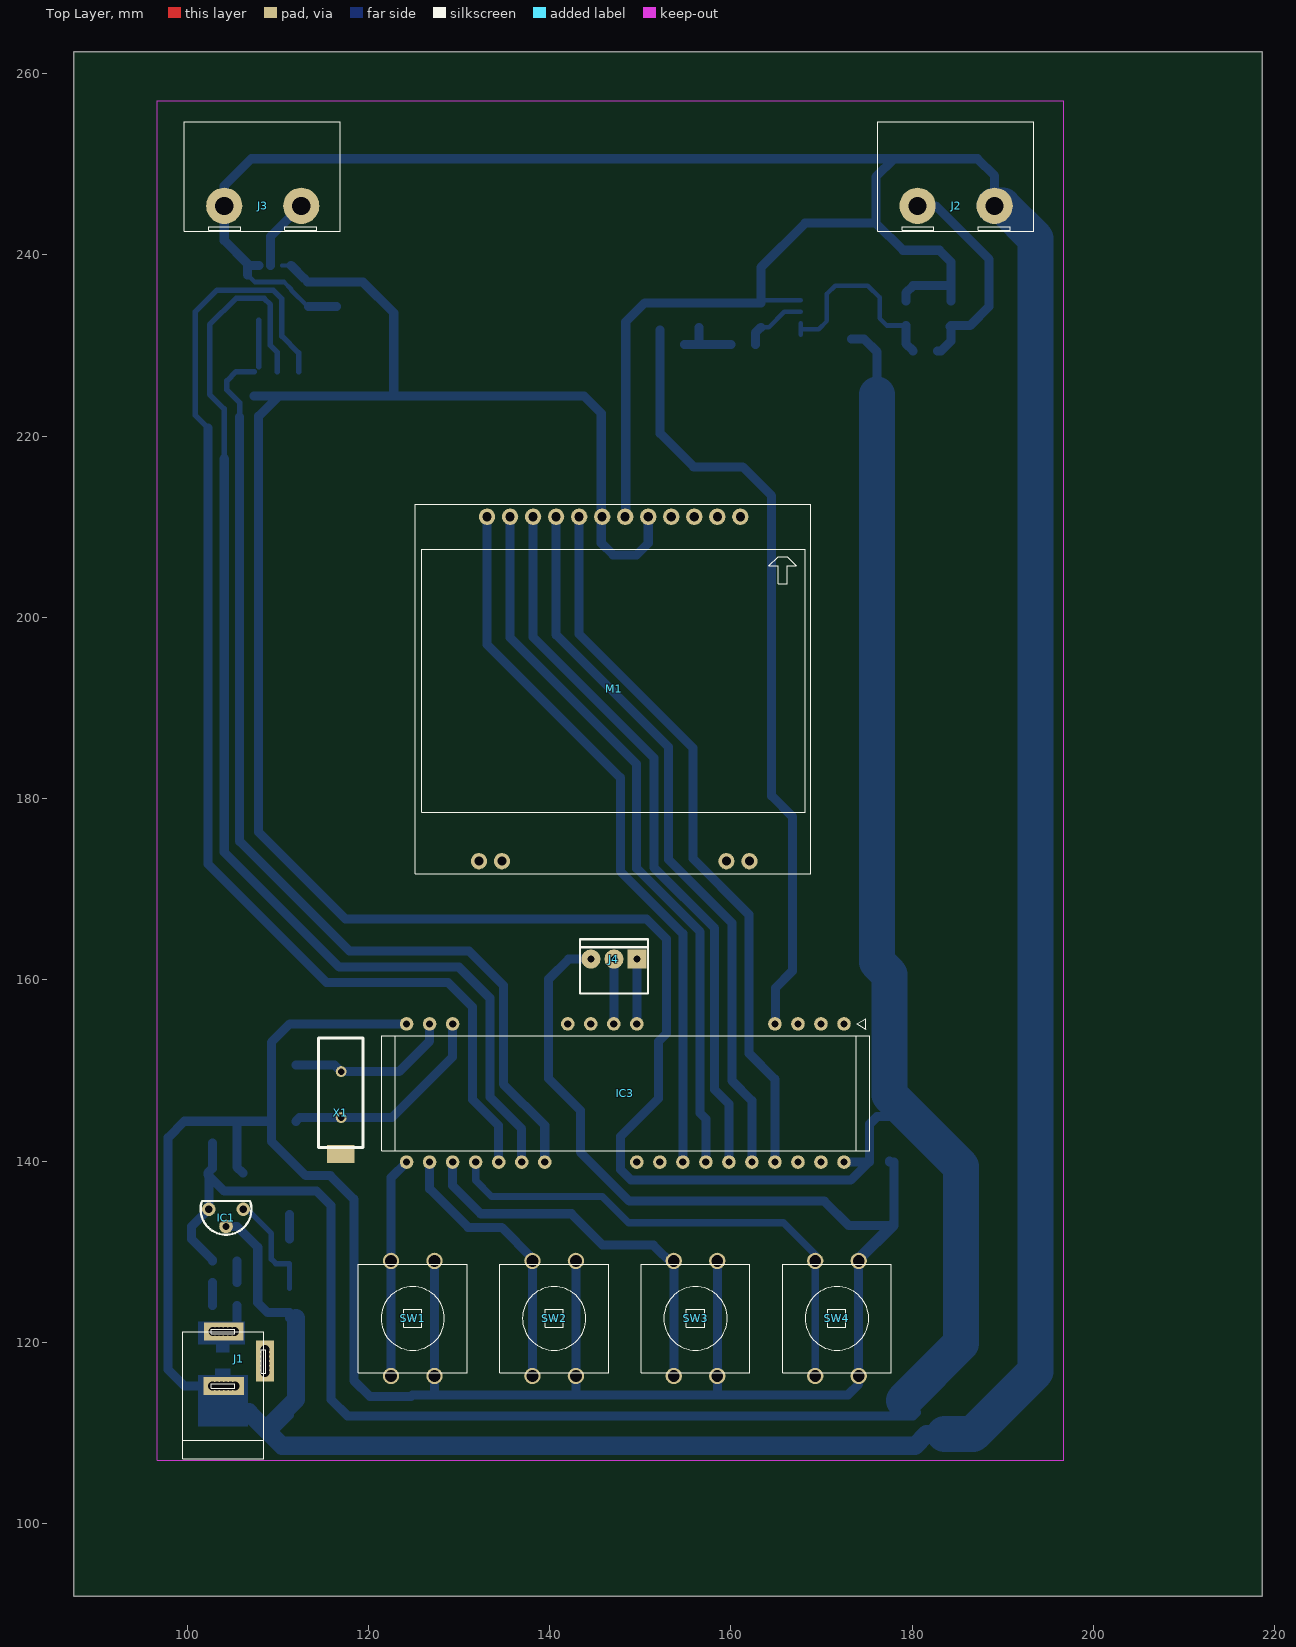
[diagram p0: Top Layer view]
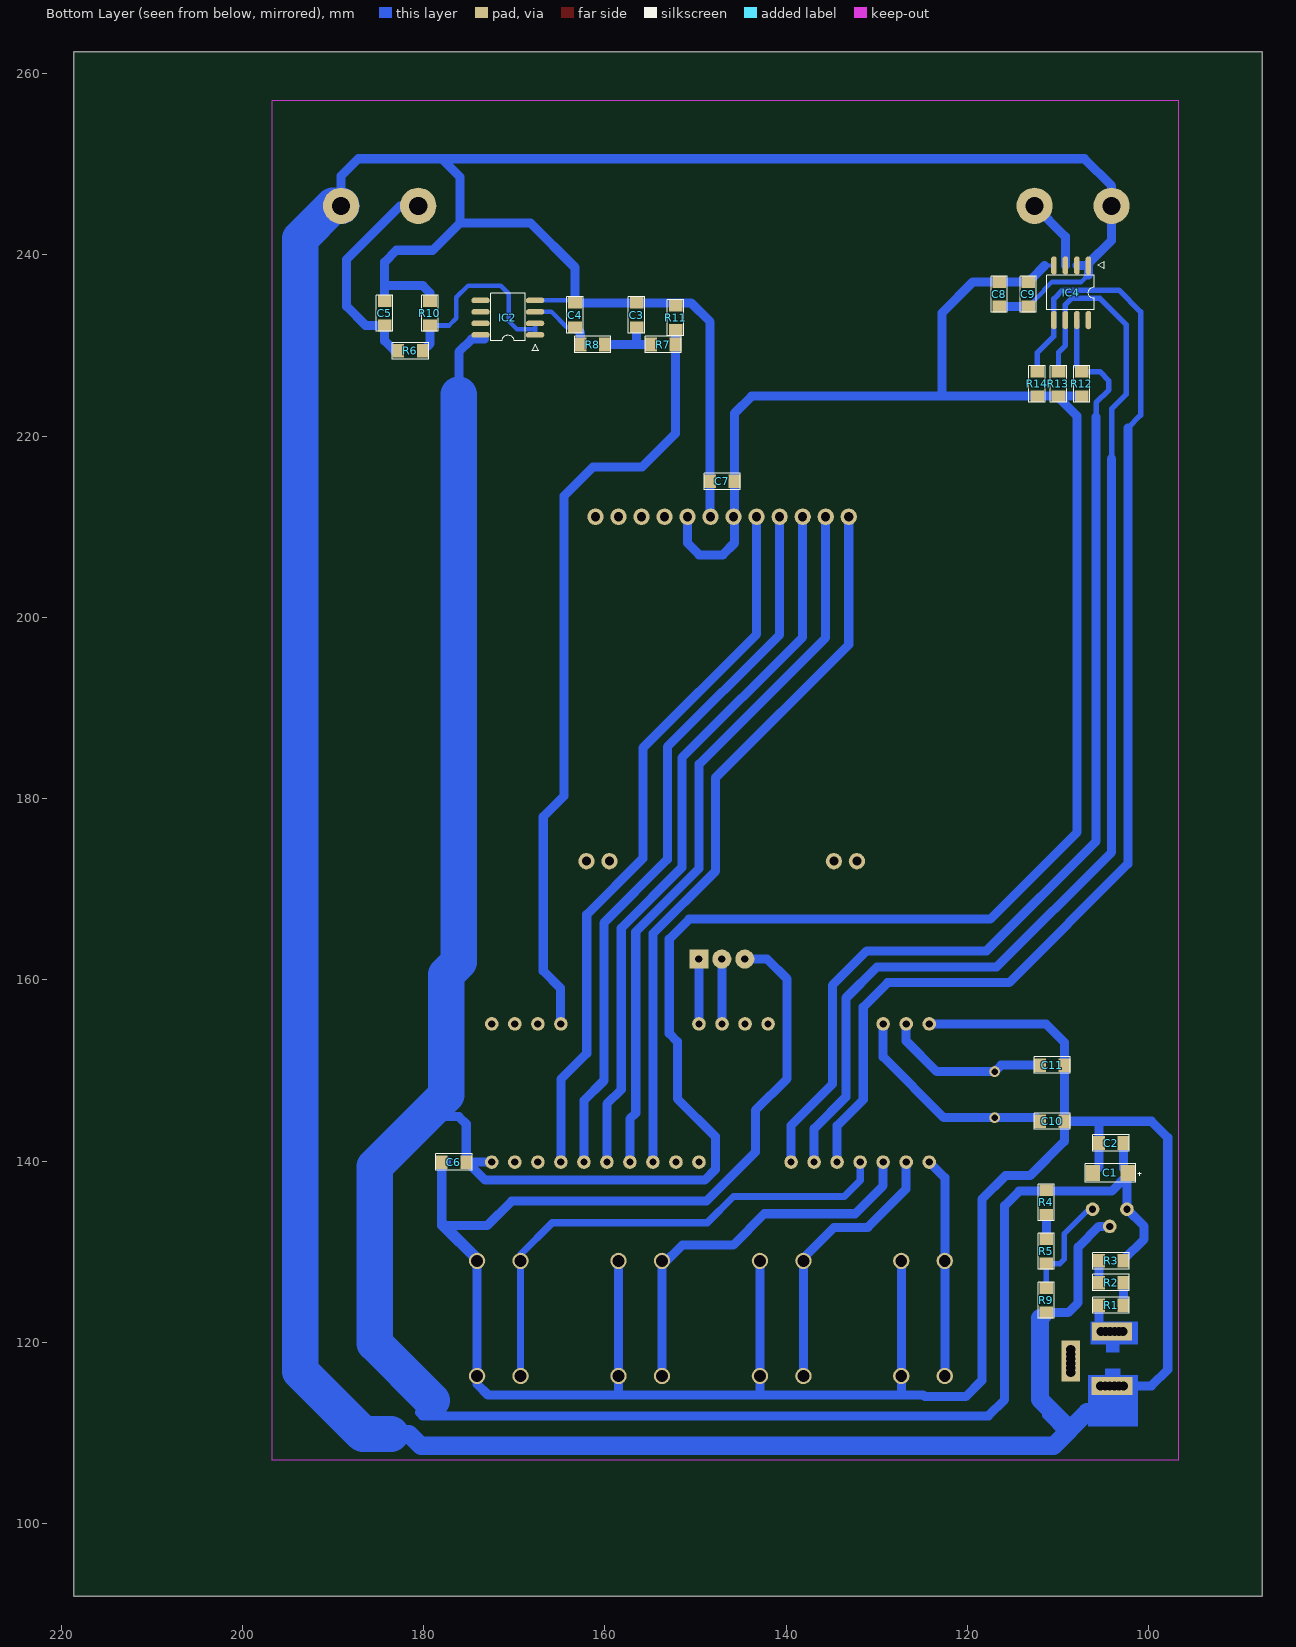
[diagram p1: Bottom Layer view, seen from below]
# Altium PCB MISC82230.PcbDoc
Units mm, origin at the board's own origin, x right, y up, seen from the top; angles counter-clockwise.
Board outline 131.1 x 170.4 mm, 2 copper layers (Top Layer, Bottom Layer); 39 components, 30 nets, 157 pads, 0 vias.

## Layer stack, top to bottom (the 12.6 mil dielectric is the usual default, probably not edited)
Top Layer: signal copper 0.0356
Dielectric: dielectric 0.32, FR-4, Dk 4.8
Bottom Layer: signal copper 0.0356

## Board outline
87.9,262.4 218.6,262.4 218.6,92 87.5,92 87.5,99.3 87.5,262.4 87.9,262.4

## Design rules (kind name [scope] priority, off if disabled: settings)
Clearance [All] p1: gap=0.2
ComponentClearance [All] p1: gap=0.254 collisioncheckmode=3 verticalgap=0.254
PolygonConnect [All] p1: connectstyle=Relief reliefconductorwidth=0.254 reliefentries=4 polygonreliefangle="90 Angle"
RoutingVias [All] p1: holewidth=0.711 width=1.27 viastyle="Through Hole" minholewidth=0.711 minwidth=1.27 maxholewidth=9 maxwidth=9
SolderMaskExpansion [All] p1: expansion=0.102
TestPointUsage [All] p1: valid=0 allowmultiple=FALSE
Testpoint [All] p1: side=15 testpointundercomponent=TRUE minsize=1.016 maxsize=2.54 preferedsize=1.524 minholesize=0 maxholesize=1.016 preferedholesize=0.813 testpointgrid=0.025 style=1023 order=0-112345678
Width [All] p1: maxlimit=9 minlimit=0.254 preferedwidth=0.3
18 further rules are at their usual default settings.

## Classes and differential pairs
component class Sheet1: C1 C2 C5 C6 C7 C8 C9 C10 C11 IC1 IC3 IC4 J1 J2 J3 J4 M1 R1 R2 R3 R4 R5 R8 R9 R10 R11 R12 R13 R14 SW1 SW2 SW3 SW4 X1

## Components (designator, comment, footprint, x,y, rotation, side; value= is the part's Value field where it differs from the comment)
C1 "10UF" C10 103.9,139.1 r0 bottom
C2 "104" 0805 102.8,142.001 r0 bottom
C3 "104" 0805 156.5,232 r90 bottom
C4 "104" 0805 163.299,232 r90 bottom
C5 "106" 0805 184.3,232.2 r90 bottom
C6 "106" 0805 175.3,139.9 r0 bottom
C7 "104" 0805 145.7,215.001 r0 bottom
C8 "106" 0805 116.5,237 r270 bottom
C9 "104" 0805 113.3,237 r270 bottom
C10 "22P" 0805 112,144.4 r180 bottom
C11 "22P" 0805 112,150.599 r180 bottom
IC1 "TL431" TO92 106.2,134.7 r180 top
IC2 "LM358/rail-to-rail" SOP8 167.675,231.13 r0 bottom
IC3 "12C5A60S2" DIP40 172.48,155.14 r180 top locked
IC4 "MAX6675" SOP8 106.63,238.845 r270 bottom
J1 "J3/5V/DC/POW" DC/POW 108.45,121.2 r270 top
J2 "0.8--4.6" SIP2/8.5 189.1,245.4 r180 top
J3 "K/IN" SIP2/8.5 112.6,245.4 r180 top
J4 "ISP" SIP3 149.156,162.511 r180 top
M1 "S/12864/LCD" S/12864/LCD 125.2,171.7 r0 top
R1 "1" 0805 102.8,124.1 r0 bottom
R2 "1" 0805 105.5,126.6 r180 bottom
R3 "1" 0805 102.8,129 r0 bottom
R4 "10" 0805 111.301,136.8 r270 bottom
R5 "10K" 0805 111.301,131.4 r270 bottom
R6 "1K" 0805 180.1,229.401 r0 bottom
R7 "10K" 0805 152.2,230.1 r0 bottom
R8 "10K" 0805 160,230.101 r0 bottom
R9 "10K" 0805 111.301,126 r270 bottom
R10 "10K" 0805 179.301,234.9 r270 bottom
R11 "100K" 0805 152.201,234.4 r270 bottom
R12 "10K" 0805 107.399,224.4 r90 bottom
R13 "10K" 0805 109.957,224.4 r90 bottom
R14 "10K" 0805 112.315,224.4 r90 bottom
SW1 "A" BUTTON/B 122.5,129 r0 top
SW2 "B" BUTTON/B 138.1,129 r0 top
SW3 "-" BUTTON/B 153.7,129 r0 top
SW4 "+" BUTTON/B 169.3,129 r0 top
X1 "12M" X 117,144.8 r90 top

## Footprints (in the part's own frame and the unit in brackets; to place one, negate y for a bottom-side part, rotate by r counter-clockwise, add the part's x,y. Pads: shape width x height; smd on the part's side, far side on the other; paste and mask are expansions set on the pad)
0805 [mm]
  rect 1.3x1.5 smd: 1(0,0) 2(2.7,0.001)
  silkscreen extent -0.65,-0.9 3.35,0.9
BUTTON/B [mm]
  round 1.8 hole 1.3: 1(0,-12.7) 1(0,0) 2(4.8,-12.7) 2(4.8,0)
  silkscreen extent -3.6,-12.35 8.4,-0.35
C10 [mm]
  rect 1.6x1.8 smd: 1(-1.6,0.4) 2(2.25,0.4)
  silkscreen extent -3.1,-0.59 3.1,1.41
DC/POW [mm]
  rect 2x2 hole 1: 1(0,-3.2) 1(0,-3.7) 1(0,-4.2) 1(0,-4.7) 1(0,-5.15) 1(0,-5.6) 2(6,-5.65) 2(6,-5.15) 2(6,-4.65) 2(6,-4.15) 2(6,-3.65) 2(6,-3.15) 3(2,0.15) 3(2.5,0.15) 3(3,0.15) 3(3.5,0.15) 3(4,0.15) 3(4.5,0.15)
  silkscreen extent -0.25,-8.95 14.05,0.25
DIP40 [mm]
  round 1.5 hole 0.8: 1(0,0) 2(2.54,0) 3(5.08,0) 4(7.62,0) 10(22.86,0) 11(25.4,0) 12(27.94,0) 13(30.48,0) 18(43.18,0) 19(45.72,0) 20(48.26,0) 21(48.26,15.24) 22(45.72,15.24) 23(43.18,15.24) 24(40.64,15.24) 25(38.1,15.24) 26(35.56,15.24) 27(33.02,15.24) 31(22.86,15.24) 32(20.32,15.24) 33(17.78,15.24) 34(15.24,15.24) 35(12.7,15.24) 36(10.16,15.24) 37(7.62,15.24) 38(5.08,15.24) 39(2.54,15.24) 40(0,15.24)
  silkscreen extent -2.85,-0.6 51,13.99
S/12864/LCD [mm]
  round 1.8 hole 1: 1(35.84,39.4) 2(33.3,39.4) 3(30.76,39.4) 4(28.22,39.4) 5(25.68,39.4) 6(23.14,39.4) 7(20.6,39.4) 8(18.06,39.4) 9(15.52,39.4) 10(12.98,39.4) 11(10.44,39.4) 12(7.9,39.4) 13(7,1.4) 14(9.54,1.4) 15(34.3,1.4) 16(36.84,1.4)
  silkscreen extent 0,0 43.6,40.8
SIP2/8.5 [mm]
  round 4 hole 2: 1(0,0) 2(8.5,0)
  silkscreen extent -4.3,-9.3 12.9,2.8
SIP3 [mm]
  rect 2.1x2.1 hole 0.813: 1(-0.484,0.211)
  round 2.1 hole 0.813: 2(2.056,0.211) 3(4.596,0.211)
  silkscreen extent -1.7,-1.99 5.8,4.01
SOP8 [mil]
  oval 80x24 smd: 1(0.99,-1.18) 2(0.99,-51.18) 3(0.99,-101.18) 4(0.99,-151.18) 5(237.99,-151.18) 6(237.99,-101.18) 7(237.99,-51.18) 8(237.99,-1.18)
  silkscreen extent -16,-181 194,67
TO92 [mm]
  round 1.5 hole 0.8 unplated: 1(0,0) 2(1.9,1.9) 3(3.8,0)
  silkscreen extent -0.9,-0.9 4.7,2.81
X [mm]
  round 1.2 hole 0.7: 1(0,0) 2(5.08,0)
  rect 2x3 smd: 3(-4.009,0.042)
  silkscreen extent -3.3,-2.4 8.78,2.5

## Part data
C1 C2 C3 C4 C5 C6 C7 C8 C9 C10 C11: library part C
IC1 IC2: library part LM358
IC3: library part 12C5A08AD
J1: library part DC/POW
J2 J3: library part J2
J4: library part J3
R1 R2 R3 R4 R5 R6 R7 R8 R9 R10 R11 R12 R13 R14: library part R
SW1 SW2 SW3 SW4: library part SW2
X1: library part X

## Nets (pads, with @x,y where several pads share a name; then routed paths per layer and width w, separated by ;. In a path a pad name is that pad's centre, name@x,y a point inside that pad or via, vN(x,y) a via of type N, cw(c..) or ccw(c..) an arc to the next point about the centre after c; other vN are vias at no path point)
0.8--4.6: C5.1 J2.2 R6.2 | length 24.4
  Bottom Layer w1: J2.2 182.6,245.4 188.5,239.5 188.5,234.3 186.4,232.2 C5.1 ; R6.2 183.2,229.4 184.3,230.5 C5.1 ; C5.1@184.2,232.1 C5.1
5.2V: J1.1 R1.2 | length 3.2
  Bottom Layer w1: J1.1@104.75,121.2 105.5,121.95 R1.2
5V: C1.1 C2.1 C6.1 C7.1 C8.1 C9.1 IC1.3 IC2.8 IC3.40 IC4.4 M1.5 M1.7 R3.1 R4.1 R12.1 R13.1 R14.1 | length 495.4
  Bottom Layer w0.4: IC4.4 111.48,238.82 ; M1.7@145.7,211.2 M1.7
  Bottom Layer w1: R3.1 102.8,129.1 100.5,131.4 100.5,132.8 IC1.3 102.4,138.6 C1.1 ; C2.1 102.8,139.2 C1.1 ; R12.1 R13.1@109.957,224.4 ; 111.48,238.82 C9.1@112.927,237.373 ; C9.1 119.4,237 122.8,233.6 122.8,224.4 ; M1.5 150.88,208.18 149.6,206.9 147,206.9 145.7,208.2 145.7,222.5 143.8,224.4 110.1,224.4 107.9,222.2 107.9,176.3 117.5,166.7 150.7,166.7 152.9,164.5 152.9,154.1 152,153.2 152,146.9 147.8,142.7 147.8,139.1 149,137.9 173.2,137.9 C6.1@175.2,139.9 ; IC3.40 C6.1 175.3,144.1 176.12,144.92 179.88,144.92 ; 173.3,230.7 174.7,230.7 176.12,229.28 176.12,224.6 ; 180.45,112.25 180.1,111.9 117.7,111.9 115.9,113.7 115.9,135.1 114.3,136.7 104.1,136.7 102.3,138.5 C1.1
  Bottom Layer w4: 176.12,224.6 176.12,161.98 177.5,160.6 177.5,147.3 185.4,139.4 185.4,119.9 179.1,113.6
GND: C1.2 C2.2 C3.2 C4.2 C5.2 C6.2 C7.2 C8.2 C9.2 C10.2 C11.2 IC1.2 IC2.4 IC3.20 IC4.1 IC4.2 J1.2 J2.1 J3.2 J4.3 M1.6 R9.2 R10.1 R11.1 SW1.2 SW2.2 SW3.2 SW4.2 | length 764
  Bottom Layer w0.5: 106.66,237.8 107.46,237 110.7,237 111.5,236.2 111.5,236.1 C9.2 C9.2@113.4,234.3 ; C4.2@163.57,234.97 IC2.4
  Bottom Layer w1: J1.2@103.3,115.2 99.7,115.2 97.9,117 97.9,142.6 99.701,144.401 C10.2 ; IC1.2 105.5,132.8 107.8,130.5 107.8,124.4 108.9,123.3 R9.2 R9.2@111.3,122.7 ; 105.5,144.301 105.5,139.35 C1.2 ; 106.66,237.8 IC4.1 ; IC4.2 IC4.1 ; 109.2,109.9 111.3,112 111.3,113 ; C9.2@113.4,234.3 C8.2 ; IC3.20 111.34,155.14 109.3,153.1 C10.2 ; SW1.2@127.3,129 127.3,114.3 127.4,114.2 ; 142.9,114.3 SW2.2@142.9,129 ; J4.3 142.1,162.3 139.9,160.1 139.9,149.1 143.4,145.6 143.4,141 148.8,135.6 170.3,135.6 173,132.9 178,132.9 ; M1.6 148.4,211.16 148.4,232.6 150.5,234.7 C4.2@163.3,234.7 ; 158.5,114.3 SW3.2@158.5,129 ; C4.2@163.3,235.24 163.3,238.6 168.2,243.5 176,243.5 ; SW4.2@174.1,129.4 178,133.3 ; C6.2@177.5,139.899 C6.2@177.5,140 ; C6.2 178,132.9 ; 178,250.6 176,248.6 176,243.5 ; R10.1 179.301,235.801 180.1,236.6 184.301,236.6 ; C5.2 184.301,239.199 183,240.5 179,240.5 176,243.5 ; J2.1 189.1,248.7 187.2,250.6 107.1,250.6 104.1,247.6 J3.2 104.1,241.6 106.66,239.04 IC4.1 ; C10.2 109.3,142.2 113.1,138.4 115.8,138.4 118.4,135.8 118.4,115.8 120.186,114.014 124.7,114.014 124.886,114.2 172.9,114.2 174.1,115.4 174.1,129 178,132.9
  Bottom Layer w2: 106.1,112.3 106.8,112.3 110.5,108.6 180.3,108.6 181.6,109.9 184.4,109.9 ; 108.9,110.4 108.9,110.6 112,113.7 R9.2@112,122.7
  Bottom Layer w4: 183.6,109.9 186.7,109.9 193.6,116.8 193.6,241.8 190,245.4 J2.1
K/CS: IC3.26 IC4.6 R13.2 | length 130.3
  Bottom Layer w0.6: 104.1,217.5 104.1,223 102.5,224.6 102.5,232.3 105.4,235.2 108.5,235.2 109.2,234.5 109.2,230 109.958,229.242 R13.2
  Bottom Layer w1: 104.1,217.5 104.1,174.1 116.8,161.4 130,161.4 133.4,158 133.4,147.1 136.92,143.58 IC3.26
K/SCK: IC3.25 IC4.5 R14.2 | length 135.3
  Bottom Layer w0.6: 102.3,220.9 100.9,222.3 100.9,233.7 103.3,236.1 109.5,236.1 110.47,235.13 110.47,231.03 112.316,229.184 R14.2
  Bottom Layer w1: 102.3,220.9 102.3,172.8 115.4,159.7 128.8,159.7 131.5,157 131.5,146.8 134.38,143.92 IC3.25
K/SO: IC3.27 IC4.7 R12.2 | length 117
  Bottom Layer w0.6: 105.8,222.1 105.8,223.7 104.4,225.1 104.4,226.1 105.4,227.1 R12.2 ; R12.2@107.93,227.63 IC4.7
  Bottom Layer w1: 105.8,222.1 105.8,175.3 117.9,163.2 131.1,163.2 134.9,159.4 134.9,148.5 139.46,143.94 IC3.27
KEY1: IC3.21 SW1.1 | length 24.3
  Bottom Layer w1: SW1.1@122.5,116.3 122.5,138.18 IC3.21
KEY2: IC3.22 SW2.1 | length 30.5
  Bottom Layer w1: IC3.22 126.76,136.94 131,132.7 134.7,132.7 138.1,129.3 SW2.1@138.1,116.3
KEY3: IC3.23 SW3.1 | length 42.8
  Bottom Layer w1: IC3.23 129.3,137.3 132.4,134.2 142.4,134.2 145.857,130.743 151.457,130.743 153.7,128.5 SW3.1@153.7,116.3
KEY4: IC3.24 SW4.1 | length 56.3
  Bottom Layer w0.8: IC3.24 131.84,137.86 133.6,136.1 145.8,136.1 148.7,133.2 165.8,133.2 169.3,129.7 SW4.1@169.3,116.3
LCD/BL: IC3.38
LCD/CS: IC3.33 M1.12 | length 80.1
  Bottom Layer w1: M1.12 133.1,197 147.8,182.3 147.8,172 154.7,165.1 IC3.33
LCD/RS: IC3.35 M1.10 | length 80.1
  Bottom Layer w1: M1.10 138.18,197.82 151.5,184.5 151.5,172.4 158.2,165.7 158.2,147.9 159.78,146.32 IC3.35
LCD/RST: IC3.34 M1.11 | length 80.1
  Bottom Layer w1: M1.11 135.64,197.76 149.6,183.8 149.6,172.3 156.6,165.3 156.6,145.3 157.24,144.66 IC3.34
LCD/SCK: IC3.37 M1.8 | length 80.1
  Bottom Layer w1: M1.8 143.26,198.14 155.8,185.6 155.8,173.4 162,167.2 162,151.9 164.86,149.04 IC3.37
LCD/SDA: IC3.36 M1.9 | length 80.1
  Bottom Layer w1: M1.9 140.72,198.08 153.1,185.7 153.1,173.3 160.1,166.3 160.1,148.9 162.32,146.68 IC3.36
NetC3_1: C3.1 R7.2 R8.1 | length 6.9
  Bottom Layer w1: R7.2 159.998,230.099 R8.1 ; 156.5,230.199 C3.1
NetC4_1: C4.1 IC2.3 R8.2 | length 7.3
  Bottom Layer w0.5: C4.1 164.2,232 165.9,233.7 IC2.3
  Bottom Layer w1: R8.2 162.7,231.402 C4.1
NetC10_1: C10.1 IC3.18 X1.1 | length 23.9
  Bottom Layer w1: C10.1 112.4,144.8 122.6,144.8 129.3,151.5 IC3.18
NetC11_1: C11.1 IC3.19 X1.2 | length 18.3
  Bottom Layer w1: C11.1 116.281,150.599 X1.2 123.38,149.88 126.76,153.26 IC3.19
NetIC1_1: IC1.1 R5.2 R9.1 | length 11.9
  Bottom Layer w0.6: IC1.1 106.6,134.7 109.3,132 109.3,129.2 109.8,128.7 R5.2 111.3,126.001 R9.1
NetIC2_1: IC2.1 IC2.2 R6.1 R10.2 | length 22.9
  Bottom Layer w0.5: IC2.1 IC2.2 ; 167.7,231.8 169.7,231.8 170.6,232.7 170.6,235.7 171.5,236.6 175.1,236.6 176.4,235.3 176.4,233 177.2,232.2 R10.2
  Bottom Layer w1: R10.2 179.3,230.202 R6.1
NetIC3_10: IC3.10 J4.1 | length 7.2
  Bottom Layer w1: IC3.10 149.64,155.16 J4.1
NetIC3_11: IC3.11 J4.2 | length 7.2
  Bottom Layer w1: IC3.11 147.1,155.16 J4.2
NetIC4_3: IC4.3 J3.1 | length 8
  Bottom Layer w1: IC4.3 109.2,242 J3.1
NetR1_1: R1.1 R2.2 | length 2.5
  Bottom Layer w1: R1.1@102.8,124.1 R2.2
NetR2_1: R2.1 R3.2 | length 2.4
  Bottom Layer w1: R2.1 R3.2
NetR4_2: R4.2 R5.1 | length 2.7
  Bottom Layer w1: R4.2 R4.2 R5.1
PWM: IC3.4 R7.1 R11.2 | length 86.6
  Bottom Layer w1: R11.2 152.2,220.3 155.9,216.6 161.3,216.6 164.5,213.4 164.5,180.3 166.8,178 166.8,161 164.9,159.1 IC3.4@164.9,155.14
pads on no net: IC2.5 IC2.6 IC2.7 IC3.1 IC3.2 IC3.3 IC3.12 IC3.13 IC3.31 IC3.32 IC3.39 IC4.8 J1.3 M1.1 M1.2 M1.3 M1.4 M1.13 M1.14 M1.15 M1.16 X1.3

## Keep-outs
Keep-Out Layer:
  lines w0.05: 96.7,107 196.7,107 196.7,257 96.7,257 96.7,107

## Other copper
Bottom Layer:
  rectangle net 5.2V: 103.2,118.9 104.7,120.7
  rectangle net 5.2V: 101.2,119.8 106.4,122.3
  rectangle net GND: 103.1,115.2 104.8,117.1
  rectangle net GND: 101.2,110.7 106.7,116.4